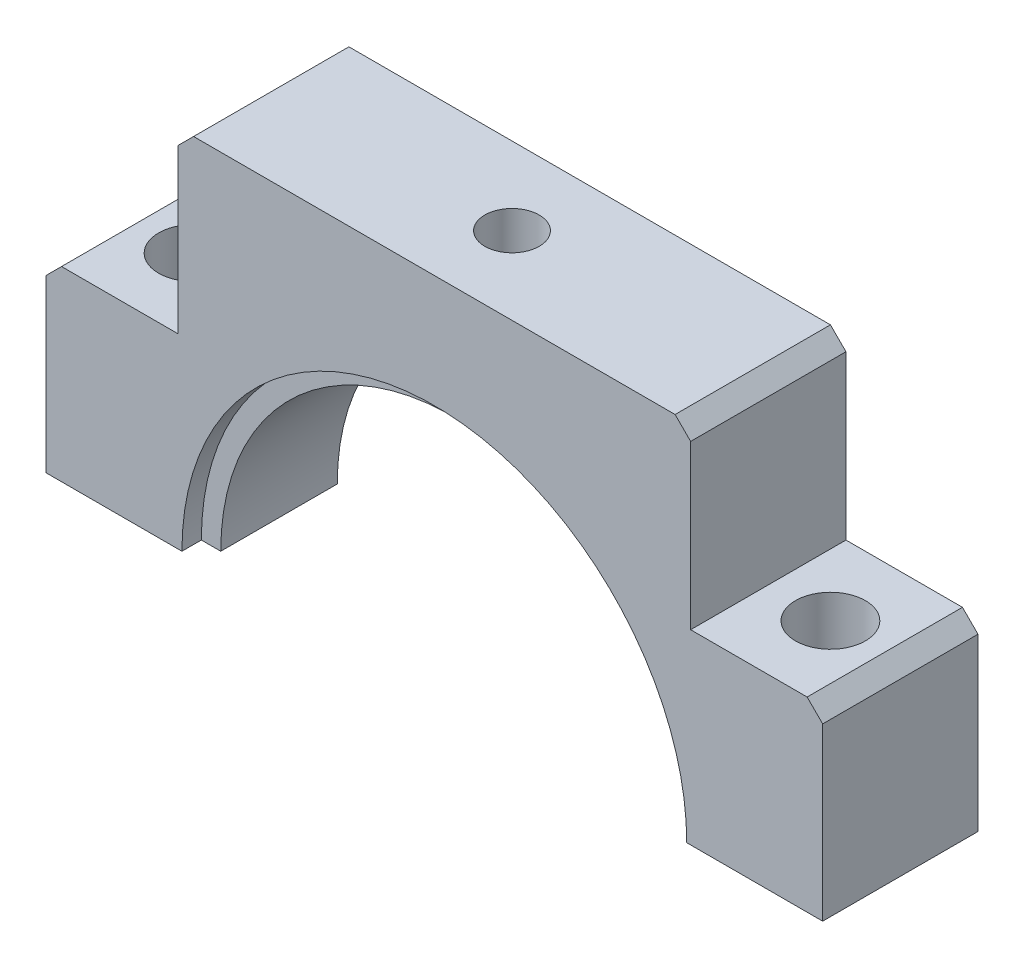
from build123d import *

# Parameters (mm, degrees)
BOSS_EXTRUDE1_DEPTH       = 20
CHAMFER1_SIZE             = 2
M8X1_0_TAPPED_HOLE1_D     = 7
M8X1_0_TAPPED_HOLE1_DEPTH = 13
M8X1_0_TAPPED_HOLE1_TIP   = 2.103012167
HOLE2_D                   = 9
SKETCH15_R                = 32.5
CUT_EXTRUDE3_DEPTH        = 2.5
CUT_EXTRUDE4_START        = -2.5
SKETCH16_R                = 32.5
CUT_EXTRUDE4_DEPTH        = 2.5
HOLE3_D                   = 4


with BuildPart() as part:
    # Sketch1 → Boss-Extrude1 (new body)
    with BuildSketch(Plane.XY):
        with BuildLine():
            Line((-50, 24), (-33, 24))
            Line((-33, 24), (-33, 47))
            Line((-33, 47), (33, 47))
            Line((33, 47), (33, 24))
            Line((33, 24), (50, 24))
            Line((50, 24), (50, 0))
            Line((50, 0), (30, 0))
            ThreePointArc((30, 0), (0, 30), (-30, 0))
            Line((-30, 0), (-50, 0))
            Line((-50, 0), (-50, 24))
        make_face()
    extrude(amount=BOSS_EXTRUDE1_DEPTH)

    # Chamfer1
    chamfer1_edges = [part.edges().sort_by_distance(p)[0] for p in [
        (-50, 24, 10),
        (-33, 47, 10),
        (33, 47, 10),
        (50, 24, 10),
    ]]
    chamfer(chamfer1_edges, length=CHAMFER1_SIZE)

    # M8x1.0 Tapped Hole1
    with Locations(Plane(origin=(0, 47, 0), x_dir=(1, 0, 0), z_dir=(0, 1, 0))):
        with Locations((0, -10)):
            Hole(M8X1_0_TAPPED_HOLE1_D / 2, depth=M8X1_0_TAPPED_HOLE1_DEPTH)
            with Locations((0, 0, -(M8X1_0_TAPPED_HOLE1_DEPTH + M8X1_0_TAPPED_HOLE1_TIP / 2))):  # 118° drill point
                Cone(0, M8X1_0_TAPPED_HOLE1_D / 2, M8X1_0_TAPPED_HOLE1_TIP, mode=Mode.SUBTRACT)

    # Hole2 (through all)
    with Locations(Plane(origin=(0, 24, 0), x_dir=(1, 0, 0), z_dir=(0, 1, 0))):
        with Locations((-41, -10), (41, -10)):
            Hole(HOLE2_D / 2)

    # Sketch15 → Cut-Extrude3 (cut)
    with BuildSketch(Plane(origin=(0, 0, 0), x_dir=(-1, 0, 0), z_dir=(0, 0, -1))):
        Circle(SKETCH15_R)
    extrude(amount=-CUT_EXTRUDE3_DEPTH, mode=Mode.SUBTRACT)

    # Sketch16 → Cut-Extrude4 (cut)
    with BuildSketch(Plane.XY.offset(20).offset(CUT_EXTRUDE4_START)):
        Circle(SKETCH16_R)
    extrude(amount=CUT_EXTRUDE4_DEPTH, mode=Mode.SUBTRACT)

    # Hole3 (through all)
    with Locations(Plane(origin=(0, 47, 0), x_dir=(1, 0, 0), z_dir=(0, 1, 0))):
        with Locations((0, -10)):
            Hole(HOLE3_D / 2)


solid = part.part
